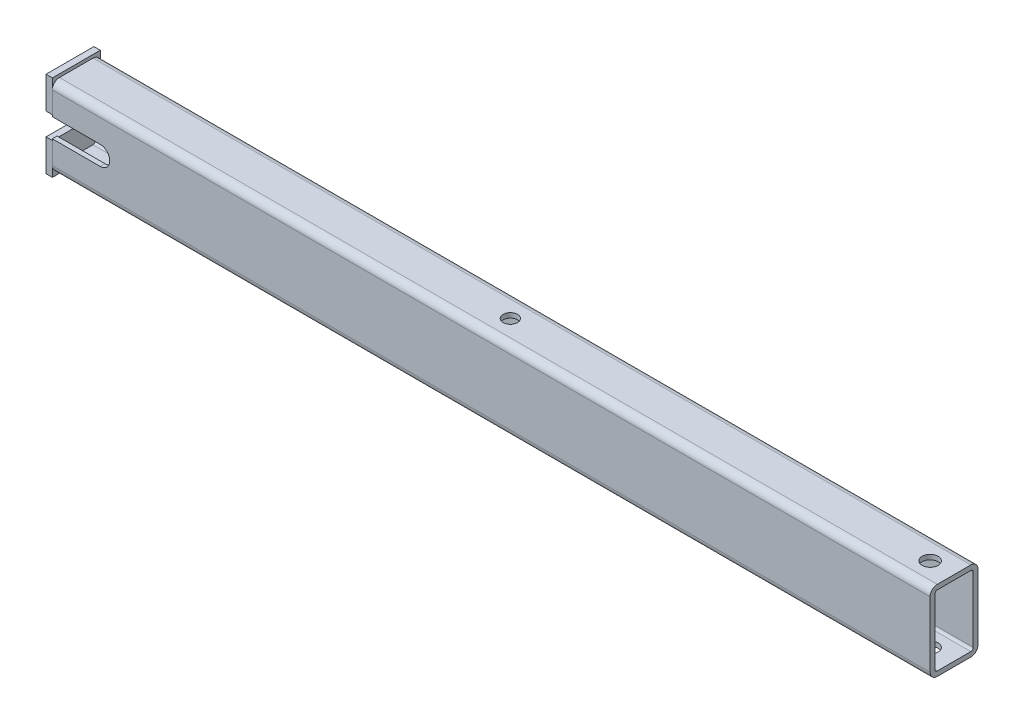
from build123d import *

# Parameters (mm, degrees)
STRUCTURAL_MEMBER2_DEPTH = 550
CUT_EXTRUDE1_DEPTH       = 321.179588302
SKETCH5_R                = 5
CUT_EXTRUDE2_DEPTH       = 50
SKETCH6_R                = 4.5
CUT_EXTRUDE3_DEPTH       = 323.048084555
SKETCH7_W                = 30
SKETCH7_H                = 20
BOSS_EXTRUDE1_DEPTH      = 4


with BuildPart() as part:
    # Sketch1 → Structural Member2 (new body)
    with BuildSketch(Plane.YZ.offset(-232.210810811)):
        with BuildLine():
            Line((-20.5, -15), (20.5, -15))
            ThreePointArc((20.5, -15), (23.681980515, -13.681980515), (25, -10.5))
            Line((25, -10.5), (25, 10.5))
            ThreePointArc((25, 10.5), (23.681980515, 13.681980515), (20.5, 15))
            Line((20.5, 15), (-20.5, 15))
            ThreePointArc((-20.5, 15), (-23.681980515, 13.681980515), (-25, 10.5))
            Line((-25, 10.5), (-25, -10.5))
            ThreePointArc((-25, -10.5), (-23.681980515, -13.681980515), (-20.5, -15))
        make_face()
        with BuildLine():
            Line((-20.5, -12), (20.5, -12))
            ThreePointArc((20.5, -12), (21.560660172, -11.560660172), (22, -10.5))
            Line((22, -10.5), (22, 10.5))
            ThreePointArc((22, 10.5), (21.560660172, 11.560660172), (20.5, 12))
            Line((20.5, 12), (-20.5, 12))
            ThreePointArc((-20.5, 12), (-21.560660172, 11.560660172), (-22, 10.5))
            Line((-22, 10.5), (-22, -10.5))
            ThreePointArc((-22, -10.5), (-21.560660172, -11.560660172), (-20.5, -12))
        make_face(mode=Mode.SUBTRACT)
    extrude(amount=STRUCTURAL_MEMBER2_DEPTH)

    # Sketch4 → Cut-Extrude1 (cut, through all)
    with BuildSketch(Plane.XY.offset(15)):
        with BuildLine():
            Line((-232.210810811, 6), (-202.210810811, 6))
            ThreePointArc((-202.210810811, 6), (-196.210810811, 0), (-202.210810811, -6))
            Line((-202.210810811, -6), (-232.210810811, -6))
            ThreePointArc((-232.210810811, -6), (-238.210810811, 0), (-232.210810811, 6))
        make_face()
    extrude(amount=-CUT_EXTRUDE1_DEPTH, mode=Mode.SUBTRACT)

    # Sketch5 → Cut-Extrude2 (cut)
    with BuildSketch(Plane(origin=(0, -25, 0), x_dir=(-1, 0, 0), z_dir=(0, -1, 0))):
        with Locations(Location((-302.789189189, 0, 0), (0, 0, 90))):
            Circle(SKETCH5_R)
    extrude(amount=-CUT_EXTRUDE2_DEPTH, mode=Mode.SUBTRACT)

    # Sketch6 → Cut-Extrude3 (cut, through all)
    with BuildSketch(Plane(origin=(0, 25, 0), x_dir=(1, 0, 0), z_dir=(0, 1, 0))):
        with Locations(Location((39.789189189, 0, 0), (0, 0, 270))):
            Circle(SKETCH6_R)
    extrude(amount=-CUT_EXTRUDE3_DEPTH, mode=Mode.SUBTRACT)


with BuildPart() as body_2:
    # Sketch7 → Boss-Extrude1 (new body)
    with BuildSketch(Plane.ZY.offset(232.210810811)):
        with Locations((-0.061159419, 17)):
            Rectangle(SKETCH7_W, SKETCH7_H)
    extrude(amount=BOSS_EXTRUDE1_DEPTH)


with BuildPart() as body_3:
    # Mirror2: mirrored copy
    add(body_2.part.mirror(Plane.ZX))


solid = Compound([part.part, body_2.part, body_3.part])
